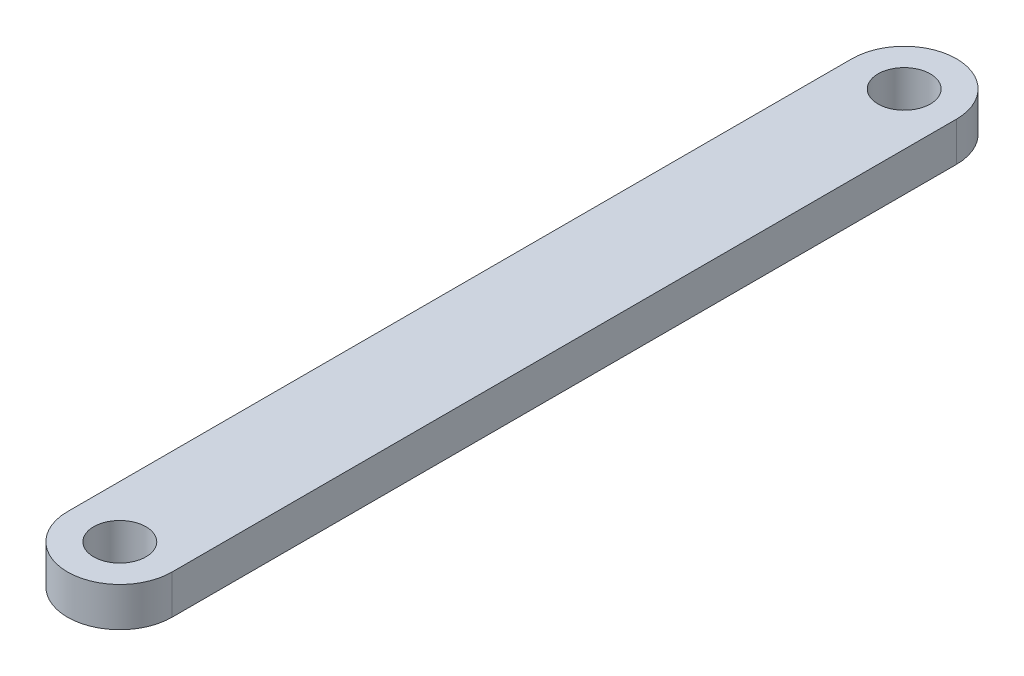
from build123d import *

# Parameters (mm, degrees)
SKETCH1_R           = 10
BOSS_EXTRUDE1_DEPTH = 15


with BuildPart() as part:
    # Sketch1 → Boss-Extrude1 (new body)
    with BuildSketch(Plane(origin=(0, 0, 0), x_dir=(1, 0, 0), z_dir=(0, 1, 0))):
        with BuildLine():
            Line((-20, 0), (-20, 300))
            ThreePointArc((-20, 300), (0, 320), (20, 300))
            Line((20, 300), (20, 0))
            ThreePointArc((20, 0), (0, -20), (-20, 0))
        make_face()
        with Locations(Location((0, 300, 0), (0, 0, 270))):
            Circle(SKETCH1_R, mode=Mode.SUBTRACT)
        with Locations(Location((0, 0, 0), (0, 0, 270))):
            Circle(SKETCH1_R, mode=Mode.SUBTRACT)
    extrude(amount=BOSS_EXTRUDE1_DEPTH)


solid = part.part
